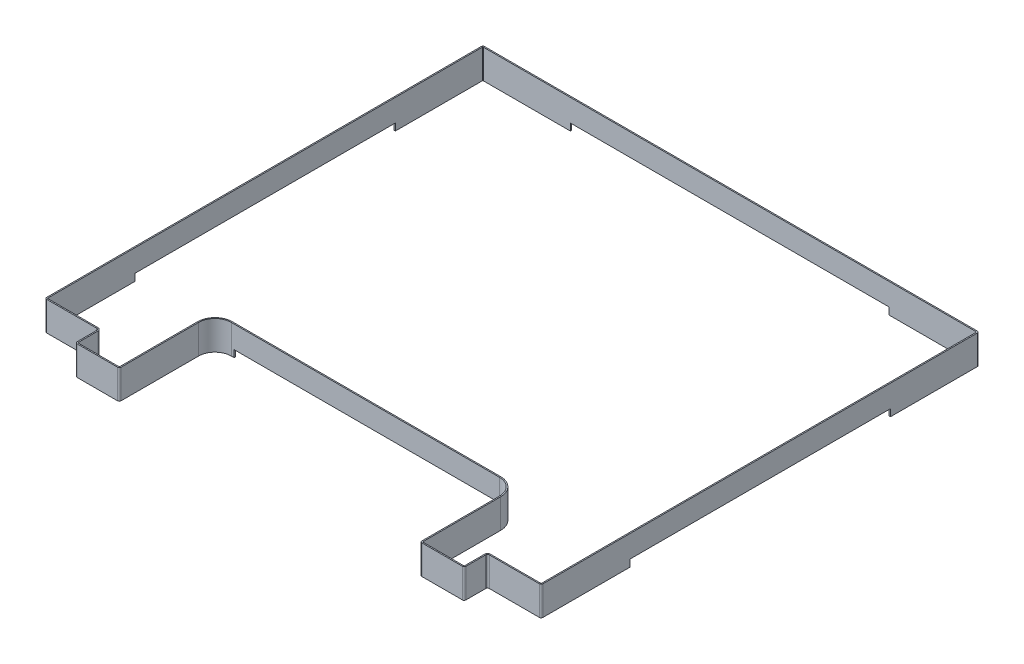
from build123d import *

# Parameters (mm, degrees)
SKETCH_1_W          = 667
SKETCH_1_H          = 791
EXTRUDE_1_DEPTH     = 50
SKETCH_6_W          = 516
SKETCH_6_H          = 164
CUT_EXTRUDE_1_DEPTH = 520.752344872
SKETCH_4_W          = 751
SKETCH_4_H          = 50
EXTRUDE_2_DEPTH     = 92
SKETCH_5_W          = 751
SKETCH_5_H          = 50
EXTRUDE_3_DEPTH     = 92
SHELL_2_T           = -2
FILLET_1_R          = 1
FILLET_2_R          = 3
FILLET_3_R          = 5
FILLET_4_R          = 28
FILLET_5_R          = 30
SKETCH_7_W          = 447
SKETCH_7_H          = 12
CUT_EXTRUDE_2_DEPTH = 2
SKETCH_8_W          = 447
SKETCH_8_H          = 12
CUT_EXTRUDE_3_DEPTH = 2
SKETCH_9_W          = 547
SKETCH_9_H          = 12
CUT_EXTRUDE_4_DEPTH = 2
SKETCH_10_W         = 450
SKETCH_10_H         = 12
CUT_EXTRUDE_5_DEPTH = 50


with BuildPart() as part:
    # 草图1 → 凸台-拉伸1 (new body)
    with BuildSketch(Plane(origin=(0, 0, 0), x_dir=(1, 0, 0), z_dir=(0, 1, 0))):
        Rectangle(SKETCH_1_W, SKETCH_1_H)
    extrude(amount=EXTRUDE_1_DEPTH)

    # 草图6 → 切除-拉伸1 (cut, through all)
    with BuildSketch(Plane(origin=(0, 50, 0), x_dir=(1, 0, 0), z_dir=(0, 1, 0))):
        with Locations((0, -313.5)):
            Rectangle(SKETCH_6_W, SKETCH_6_H)
    extrude(amount=-CUT_EXTRUDE_1_DEPTH, mode=Mode.SUBTRACT)

    # 草图4 → 凸台-拉伸2 (add)
    with BuildSketch(Plane(origin=(333.5, 0, 0), x_dir=(0, 0, -1), z_dir=(1, 0, 0))):
        with Locations((20, 25)):
            Rectangle(SKETCH_4_W, SKETCH_4_H)
    extrude(amount=EXTRUDE_2_DEPTH)

    # 草图5 → 凸台-拉伸3 (add)
    with BuildSketch(Plane.ZY.offset(333.5)):
        with Locations((-20, 25)):
            Rectangle(SKETCH_5_W, SKETCH_5_H)
    extrude(amount=EXTRUDE_3_DEPTH)

    # 抽壳2
    shell_2_openings = [part.faces().sort_by_distance(p)[0] for p in [
        (0, 50, -50.405146974),
        (0, 0, -50.405146974),
    ]]
    offset(amount=SHELL_2_T, openings=shell_2_openings, kind=Kind.INTERSECTION)

    # 圆角1
    fillet_1_edges = [part.edges().sort_by_distance(p)[0] for p in [
        (331.5, 25, 393.5),
        (-260, 25, 393.5),
        (-331.5, 25, 393.5),
        (260, 25, 393.5),
        (423.5, 25, 353.5),
        (423.5, 25, -393.5),
        (-423.5, 25, -393.5),
        (-423.5, 25, 353.5),
    ]]
    fillet(fillet_1_edges, radius=FILLET_1_R)

    # 圆角2
    fillet_2_edges = [part.edges().sort_by_distance(p)[0] for p in [
        (-333.5, 25, 355.5),
        (333.5, 25, 355.5),
        (425.5, 25, 355.5),
        (425.5, 25, -395.5),
        (-425.5, 25, -395.5),
        (-425.5, 25, 355.5),
        (333.5, 25, 395.5),
        (-333.5, 25, 395.5),
        (258, 25, 395.5),
        (-258, 25, 395.5),
    ]]
    fillet(fillet_2_edges, radius=FILLET_2_R)

    # 圆角3
    fillet_3_edges = [part.edges().sort_by_distance(p)[0] for p in [
        (331.5, 25, 353.5),
        (-331.5, 25, 353.5),
    ]]
    fillet(fillet_3_edges, radius=FILLET_3_R)

    # 圆角4
    fillet_4_edges = [part.edges().sort_by_distance(p)[0] for p in [
        (-258, 25, 231.5),
        (258, 25, 231.5),
    ]]
    fillet(fillet_4_edges, radius=FILLET_4_R)

    # 圆角5
    fillet_5_edges = [part.edges().sort_by_distance(p)[0] for p in [
        (-260, 25, 229.5),
        (260, 25, 229.5),
    ]]
    fillet(fillet_5_edges, radius=FILLET_5_R)

    # 草图7 → 切除-拉伸2 (cut)
    with BuildSketch(Plane(origin=(425.5, 0, 0), x_dir=(0, 0, -1), z_dir=(1, 0, 0))):
        with Locations((20, 6)):
            Rectangle(SKETCH_7_W, SKETCH_7_H)
    extrude(amount=-CUT_EXTRUDE_2_DEPTH, mode=Mode.SUBTRACT)

    # 草图8 → 切除-拉伸3 (cut)
    with BuildSketch(Plane.ZY.offset(425.5)):
        with Locations((-20, 6)):
            Rectangle(SKETCH_8_W, SKETCH_8_H)
    extrude(amount=-CUT_EXTRUDE_3_DEPTH, mode=Mode.SUBTRACT)

    # 草图9 → 切除-拉伸4 (cut)
    with BuildSketch(Plane(origin=(0, 0, -395.5), x_dir=(-1, 0, 0), z_dir=(0, 0, -1))):
        with Locations((0, 6)):
            Rectangle(SKETCH_9_W, SKETCH_9_H)
    extrude(amount=-CUT_EXTRUDE_4_DEPTH, mode=Mode.SUBTRACT)

    # 草图10 → 切除-拉伸5 (cut, symmetric)
    with BuildSketch(Plane.XY.offset(231.5)):
        with Locations((0, 6)):
            Rectangle(SKETCH_10_W, SKETCH_10_H)
    extrude(amount=CUT_EXTRUDE_5_DEPTH, both=True, mode=Mode.SUBTRACT)


solid = part.part
